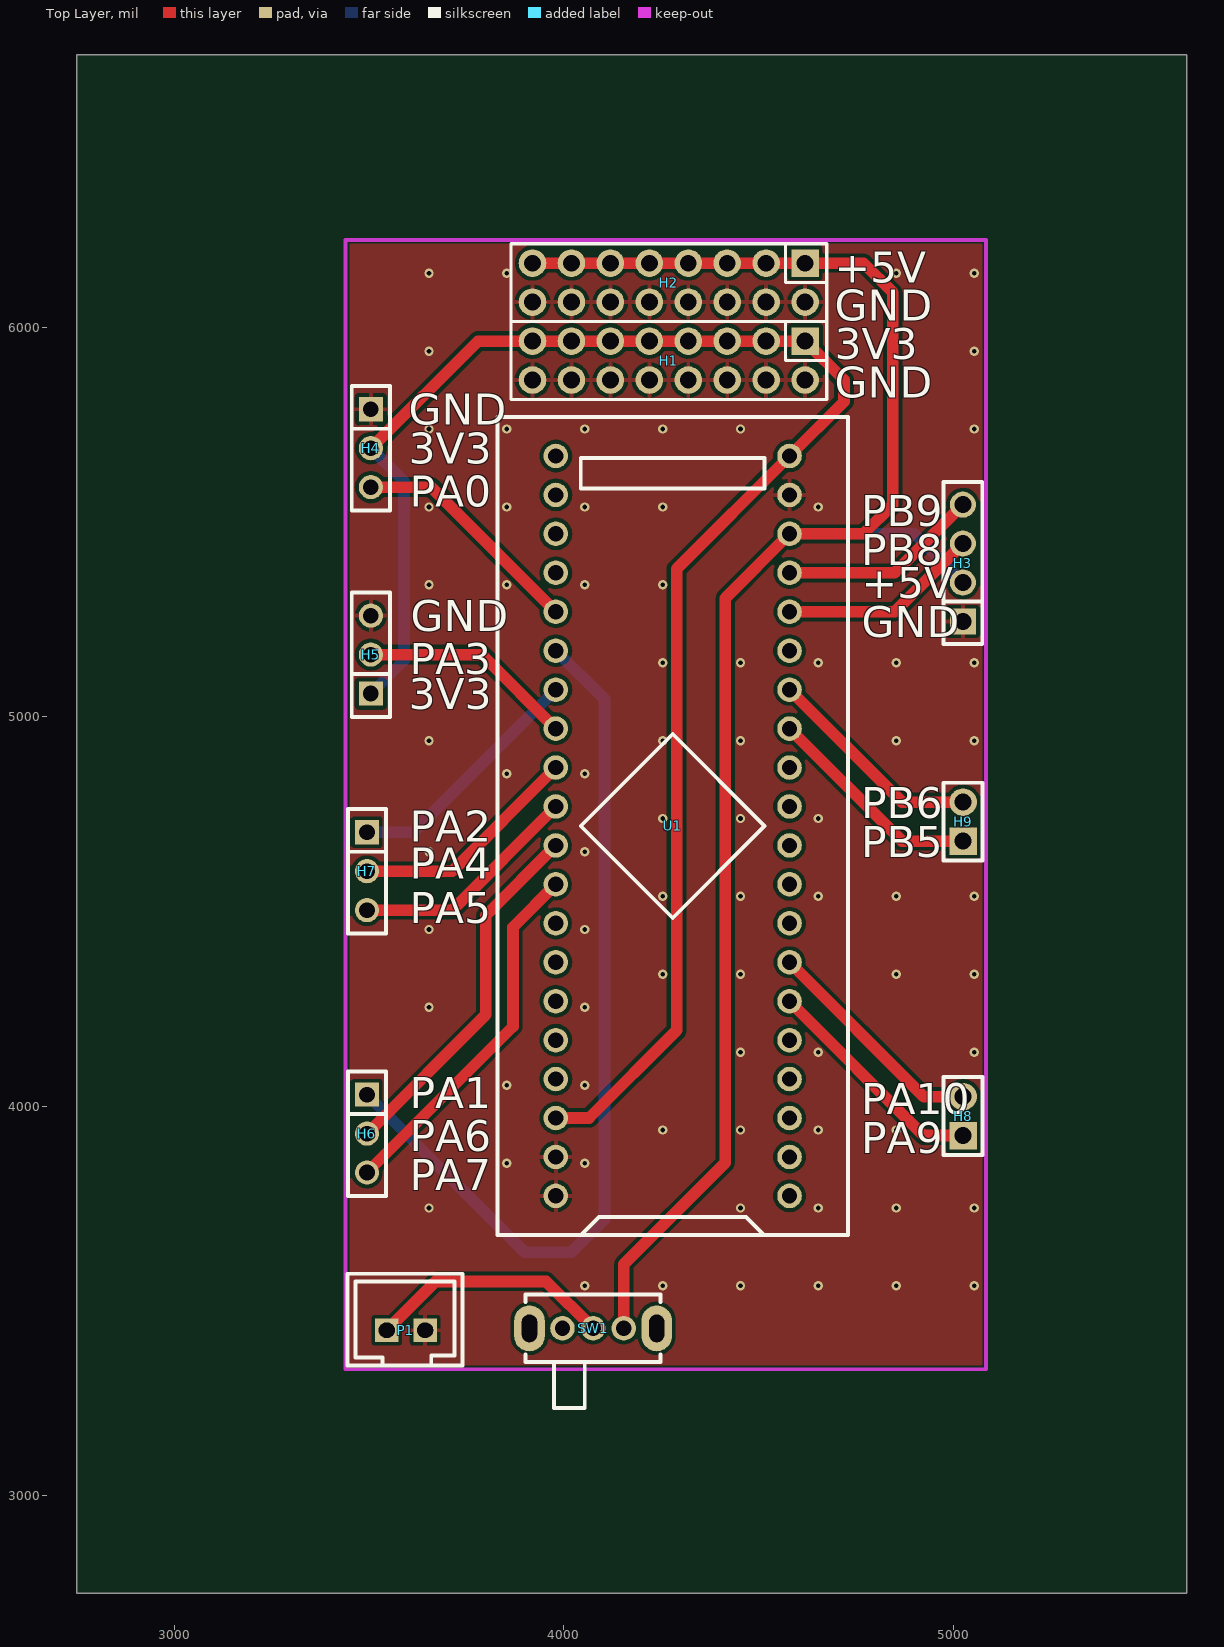
[diagram p0: Top Layer view]
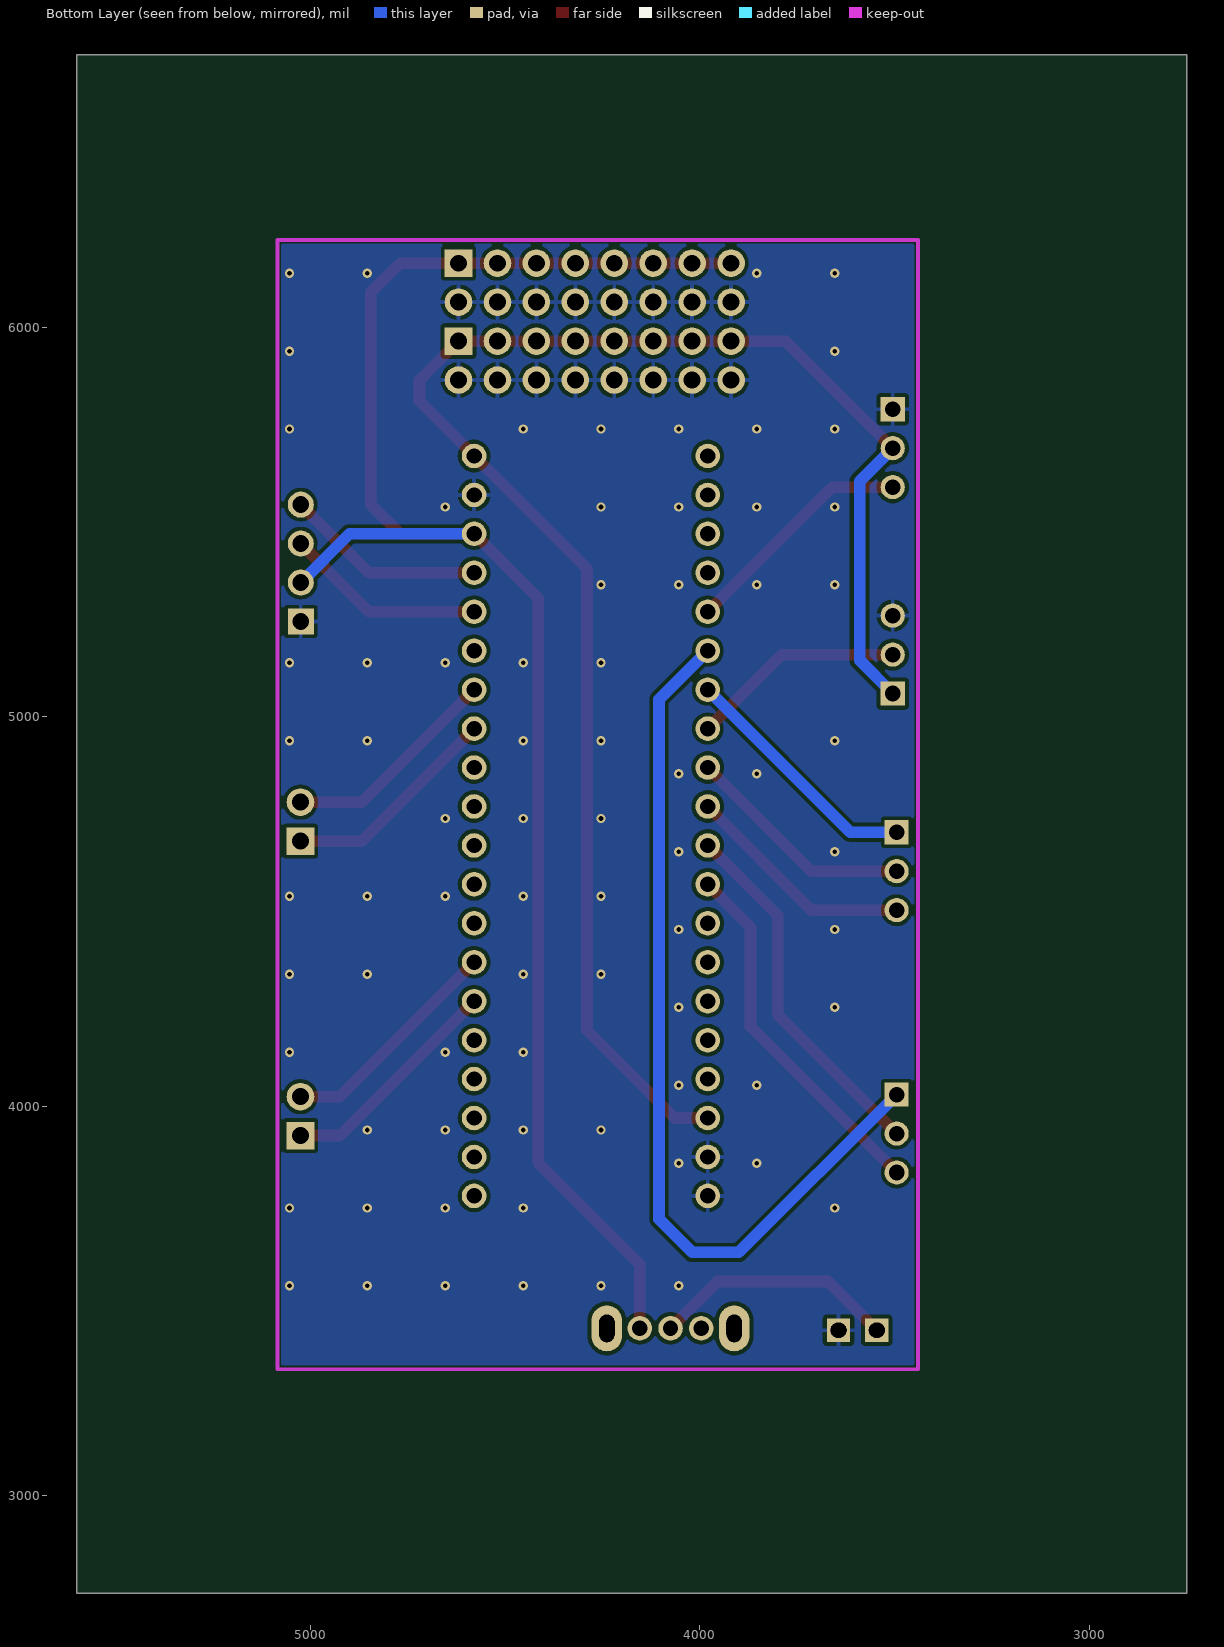
[diagram p1: Bottom Layer view, seen from below]
# Altium PCB MISC51854.pcbdoc
Units mil, origin at the board's own origin, x right, y up, seen from the top; angles counter-clockwise.
Board outline 2850 x 3950 mil, 2 copper layers (Top Layer, Bottom Layer), stack 62.206 mil thick; 12 components, 38 nets, 99 pads, 73 vias.

## Layer stack, top to bottom
Top Solder Mask Layer: solder mask 0.394, Dk 3.3
Top Layer: signal copper 1.379
Dielectric1: surface 59.449, FR4, Dk 4.5
Bottom Layer: signal copper 1.378
Bottom Solder Mask Layer: solder mask 0.394, Dk 3.3

## Board outline
5600,2750 2750,2750 2750,6700 5600,6700

## Design rules (kind name [scope] priority, off if disabled: settings)
BoardOutlineClearance copperThickness2oz_1 [All] p2 off: genericclearance=7.99 ignorepadtopadclearanceinfootprint=FALSE except(0: Arc-SplitContinuation Track-SplitContinuation SMDPad-SplitContinuation THPad-SplitContinuation Via-SplitContinuation Fill-SplitContinuation Region-SplitContinuation Poly-SplitContinuation Text-SplitContinuation Hole-SplitContinuation; 5.98: Arc-CutoutEdge Track-CutoutEdge SMDPad-CutoutEdge THPad-CutoutEdge Via-CutoutEdge Text-CutoutEdge; 6.9: Hole-OutlineEdge Hole-CutoutEdge; 10: Poly-OutlineEdge Poly-CutoutEdge; 11.81: Arc-OutlineEdge Track-OutlineEdge SMDPad-OutlineEdge THPad-OutlineEdge Via-OutlineEdge Fill-OutlineEdge Region-OutlineEdge Text-OutlineEdge Fill-CutoutEdge Region-CutoutEdge)
BoardOutlineClearance Plane_innerPlane_1 [All] p4 off: genericclearance=4.02 ignorepadtopadclearanceinfootprint=FALSE except(0: Arc-SplitContinuation Track-SplitContinuation SMDPad-SplitContinuation THPad-SplitContinuation Via-SplitContinuation Fill-SplitContinuation Region-SplitContinuation Poly-SplitContinuation Text-SplitContinuation Hole-SplitContinuation; 5.98: Arc-CutoutEdge Track-CutoutEdge SMDPad-CutoutEdge THPad-CutoutEdge Via-CutoutEdge Text-CutoutEdge; 6.9: Hole-OutlineEdge Hole-CutoutEdge; 10: Poly-OutlineEdge Poly-CutoutEdge; 11.81: Arc-OutlineEdge Track-OutlineEdge SMDPad-OutlineEdge THPad-OutlineEdge Via-OutlineEdge Fill-OutlineEdge Region-OutlineEdge Text-OutlineEdge Fill-CutoutEdge Region-CutoutEdge)
BoardOutlineClearance Copper_copperRegion_1 [All] p6 off: genericclearance=4.02 ignorepadtopadclearanceinfootprint=FALSE except(0: Arc-SplitContinuation Track-SplitContinuation SMDPad-SplitContinuation THPad-SplitContinuation Via-SplitContinuation Fill-SplitContinuation Region-SplitContinuation Poly-SplitContinuation Text-SplitContinuation Hole-SplitContinuation; 5.98: Arc-CutoutEdge Track-CutoutEdge SMDPad-CutoutEdge THPad-CutoutEdge Via-CutoutEdge Text-CutoutEdge; 6.9: Hole-OutlineEdge Hole-CutoutEdge; 10: Poly-OutlineEdge Poly-CutoutEdge; 11.81: Arc-OutlineEdge Track-OutlineEdge SMDPad-OutlineEdge THPad-OutlineEdge Via-OutlineEdge Fill-OutlineEdge Region-OutlineEdge Text-OutlineEdge Fill-CutoutEdge Region-CutoutEdge)
BoardOutlineClearance copperThickness1oz_1 [All] p8: genericclearance=4.02 ignorepadtopadclearanceinfootprint=FALSE except(0: Arc-SplitContinuation Track-SplitContinuation SMDPad-SplitContinuation THPad-SplitContinuation Via-SplitContinuation Fill-SplitContinuation Region-SplitContinuation Poly-SplitContinuation Text-SplitContinuation Hole-SplitContinuation; 5.98: Arc-CutoutEdge Track-CutoutEdge SMDPad-CutoutEdge THPad-CutoutEdge Via-CutoutEdge Text-CutoutEdge; 6.9: Hole-OutlineEdge Hole-CutoutEdge; 10: Poly-OutlineEdge Poly-CutoutEdge; 11.81: Arc-OutlineEdge Track-OutlineEdge SMDPad-OutlineEdge THPad-OutlineEdge Via-OutlineEdge Fill-OutlineEdge Region-OutlineEdge Text-OutlineEdge Fill-CutoutEdge Region-CutoutEdge)
Clearance copperThickness2oz [All] p1 off: gap=7.99 ignorepadtopadclearanceinfootprint=FALSE except(5.98: SMDPad-Track SMDPad-SMDPad THPad-Track SMDPad-THPad THPad-THPad Track-Via SMDPad-Via THPad-Via Via-Via Fill-SMDPad Region-SMDPad Fill-THPad Region-THPad Fill-Via Region-Via Fill-Fill Fill-Region Region-Region Arc-Track Arc-SMDPad Arc-THPad Arc-Via Fill-Arc Region-Arc Arc-Arc Text-Track SMDPad-Text Text-THPad Text-Via Fill-Text Region-Text Arc-Text Text-Text; 6.9: Hole-Track Hole-SMDPad Hole-THPad Hole-Via Fill-Hole Region-Hole Hole-Arc Hole-Text; 10: Poly-Track Poly-SMDPad Poly-THPad Poly-Via Poly-Fill Poly-Region Poly-Poly Poly-Arc Poly-Text Poly-Hole; 11.81: Fill-Track Region-Track)
Clearance Plane_innerPlane [All] p3 off: gap=4.02 ignorepadtopadclearanceinfootprint=FALSE except(5.98: SMDPad-Track SMDPad-SMDPad THPad-Track SMDPad-THPad THPad-THPad Track-Via SMDPad-Via THPad-Via Via-Via Fill-SMDPad Region-SMDPad Fill-THPad Region-THPad Fill-Via Region-Via Fill-Fill Fill-Region Region-Region Arc-Track Arc-SMDPad Arc-THPad Arc-Via Fill-Arc Region-Arc Arc-Arc Text-Track SMDPad-Text Text-THPad Text-Via Fill-Text Region-Text Arc-Text Text-Text; 6.9: Hole-Track Hole-SMDPad Hole-THPad Hole-Via Fill-Hole Region-Hole Hole-Arc Hole-Text; 10: Poly-Track Poly-SMDPad Poly-THPad Poly-Via Poly-Fill Poly-Region Poly-Poly Poly-Arc Poly-Text Poly-Hole; 11.81: Fill-Track Region-Track)
Clearance Copper_copperRegion [All] p5 off: gap=4.02 ignorepadtopadclearanceinfootprint=FALSE except(5.98: SMDPad-Track SMDPad-SMDPad THPad-Track SMDPad-THPad THPad-THPad Track-Via SMDPad-Via THPad-Via Via-Via Fill-SMDPad Region-SMDPad Fill-THPad Region-THPad Fill-Via Region-Via Fill-Fill Fill-Region Region-Region Arc-Track Arc-SMDPad Arc-THPad Arc-Via Fill-Arc Region-Arc Arc-Arc Text-Track SMDPad-Text Text-THPad Text-Via Fill-Text Region-Text Arc-Text Text-Text; 6.9: Hole-Track Hole-SMDPad Hole-THPad Hole-Via Fill-Hole Region-Hole Hole-Arc Hole-Text; 10: Poly-Track Poly-SMDPad Poly-THPad Poly-Via Poly-Fill Poly-Region Poly-Poly Poly-Arc Poly-Text Poly-Hole; 11.81: Fill-Track Region-Track)
Clearance copperThickness1oz [All] p7: gap=4.02 ignorepadtopadclearanceinfootprint=FALSE except(5.98: SMDPad-Track SMDPad-SMDPad THPad-Track SMDPad-THPad THPad-THPad Track-Via SMDPad-Via THPad-Via Via-Via Fill-SMDPad Region-SMDPad Fill-THPad Region-THPad Fill-Via Region-Via Fill-Fill Fill-Region Region-Region Arc-Track Arc-SMDPad Arc-THPad Arc-Via Fill-Arc Region-Arc Arc-Arc Text-Track SMDPad-Text Text-THPad Text-Via Fill-Text Region-Text Arc-Text Text-Text; 6.9: Hole-Track Hole-SMDPad Hole-THPad Hole-Via Fill-Hole Region-Hole Hole-Arc Hole-Text; 10: Poly-Track Poly-SMDPad Poly-THPad Poly-Via Poly-Fill Poly-Region Poly-Poly Poly-Arc Poly-Text Poly-Hole; 11.81: Fill-Track Region-Track)
DiffPairsRouting differentialPair [All] p1: maxlimit=6 minlimit=6 mostfreqgap=6 toplayer_minwidth=5 toplayer_prefwidth=10 toplayer_maxwidth=100 toplayer_mingap=6 toplayer_prefgap=6 toplayer_maxgap=6 bottomlayer_minwidth=5 bottomlayer_prefwidth=10 bottomlayer_maxwidth=100 bottomlayer_mingap=6 bottomlayer_prefgap=6 bottomlayer_maxgap=6 maxuncoupledlength=10
HoleToHoleClearance otherClearance [All] p1: gap=11.81 allowstackedmicrovias=TRUE
Length netLength [All] p1: minlimit=0 maxlimit=0
PasteMaskExpansion pasteMaskExpansion [All] p1: expansion=0
PlaneConnect innerPlane [All] p1: planeconnectstyle=Relief reliefexpansion=20 reliefentries=4 reliefconductorwidth=10 reliefairgap=10
PolygonConnect copperRegion [All] p1: connectstyle=Relief reliefconductorwidth=10 reliefentries=4 polygonreliefangle="90 Angle" airgapwidth=10 via.connectstyle=Relief via.reliefconductorwidth=10 via.reliefentries=4 via.polygonreliefangle="90 Angle" via.airgapwidth=10
RoutingVias viaSize [All] p1: holewidth=12.01 width=24.02 viastyle="Through Hole" minholewidth=11.81 minwidth=19.68 maxholewidth=248.03 maxwidth=393.7
SolderMaskExpansion solderMaskExpansion [IsVia] p1: expansion=-1000 istentingtop=TRUE
SolderMaskExpansion solderMaskExpansion [All] p2: expansion=2 istentingtop=FALSE
Width copperThickness2oz_2 [All] p1 off: maxlimit=100 minlimit=8 preferedwidth=10
Width copperThickness1oz_2 [All] p2: maxlimit=100 minlimit=5 preferedwidth=10

## Components (designator, comment, footprint, x,y, rotation, side; value= is the part's Value field where it differs from the comment)
H1 "" HDR-TH_16P-P2.54-V-F-R2-C8-S2.54-1 4270,5915 r180 top
H2 "" HDR-TH_16P-P2.54-V-F-R2-C8-S2.54-1 4270,6115 r180 top
H3 "" HDR-TH_4P-P2.54-V-F 5025,5395 r90 top
H4 "" HDR-TH_3P-P2.54-V-F 3505,5690 r270 top
H5 "" HDR-TH_3P-P2.54-V-F 3505,5160 r90 top
H6 "" HDR-TH_3P-P2.54-V-F 3495,3930 r270 top
H7 "" HDR-TH_3P-P2.54-V-F 3495,4603.81 r270 top
H8 "" HDR-TH_2P-P2.54-V-M-1 5025.79,3974.94 r90 top
H9 "" HDR-TH_2P-P2.54-V-M-1 5025.79,4731.03 r90 top
P1 "XH2.54直插座-2P" CONN-TH_XH2.54-2P 3595,3425 r0 top
SW1 "" 拨动开关_侧 4075.57,3429.94 r0 top
U1 "STM32F103C8T6-Card" CONN-TH_L53.3-W22.9_STM32F103C8T6-CARD 4280,4720 r90 top

## Footprints (in the part's own frame and the unit in brackets; to place one, negate y for a bottom-side part, rotate by r counter-clockwise, add the part's x,y. Pads: shape width x height; smd on the part's side, far side on the other; paste and mask are expansions set on the pad)
CONN-TH_L53.3-W22.9_STM32F103C8T6-CARD [mm]
  round 1.6 hole 1: 1(-24.13,-7.62) 2(-21.59,-7.62) 3(-19.05,-7.62) 4(-16.51,-7.62) 5(-13.97,-7.62) 6(-11.43,-7.62) 7(-8.89,-7.62) 8(-6.35,-7.62) 9(-3.81,-7.62) 10(-1.27,-7.62) 11(1.27,-7.62) 12(3.81,-7.62) 13(6.35,-7.62) 14(8.89,-7.62) 15(11.43,-7.62) 16(13.97,-7.62) 17(16.51,-7.62) 18(19.05,-7.62) 19(21.59,-7.62) 20(24.13,-7.62) 21(24.13,7.62) 22(21.59,7.62) 23(19.05,7.62) 24(16.51,7.62) 25(13.97,7.62) 26(11.43,7.62) 27(8.89,7.62) 28(6.35,7.62) 29(3.81,7.62) 30(1.27,7.62) 31(-1.27,7.62) 32(-3.81,7.62) 33(-6.35,7.62) 34(-8.89,7.62) 35(-11.43,7.62) 36(-13.97,7.62) 37(-16.51,7.62) 38(-19.05,7.62) 39(-21.59,7.62) 40(-24.13,7.62)
  silkscreen extent -26.67,-11.43 26.67,11.43
CONN-TH_XH2.54-2P [mil]
  rect 60x60 hole 39.37 slot 41.34 at 0 deg paste+0 mask+1.97: 1(-49.22,0) 2(49.21,0)
  silkscreen extent -150,-90 145,145
HDR-TH_2P-P2.54-V-M-1 [mm]
  rect 1.8x1.8 hole 1.1: 1(-1.27,0)
  round 1.8 hole 1.1: 2(1.27,0)
  silkscreen extent -2.54,-1.27 2.54,1.27
HDR-TH_3P-P2.54-V-F [mil]
  rect 62x62 hole 40.16: 1(-100,0)
  round 62 hole 40.16: 2(0,0) 3(100,0)
  silkscreen extent -160,-49 160,49
HDR-TH_4P-P2.54-V-F [mm]
  rect 1.7x1.7 hole 1.1: 1(-3.81,0)
  round 1.7 hole 1.1: 2(-1.27,0) 3(1.27,0) 4(3.81,0)
  silkscreen extent -5.29,-1.27 5.29,1.27
HDR-TH_16P-P2.54-V-F-R2-C8-S2.54-1 [mm]
  rect 1.8x1.8 hole 1.1: 1(-8.89,-1.27)
  round 1.8 hole 1.1: 2(-8.89,1.27) 3(-6.35,-1.27) 4(-6.35,1.27) 5(-3.81,-1.27) 6(-3.81,1.27) 7(-1.27,-1.27) 8(-1.27,1.27) 9(1.27,-1.27) 10(1.27,1.27) 11(3.81,-1.27) 12(3.81,1.27) 13(6.35,-1.27) 14(6.35,1.27) 15(8.89,-1.27) 16(8.89,1.27)
  silkscreen extent -10.3,-2.54 10.3,2.54
拨动开关_侧 [mil]
  round 63 hole 39.4 paste+0 mask+2: 1(-78.7,0) 2(0,0) 3(78.7,0)
  oval 78.7x118.1 hole 39.4 slot 70.9 at 90 deg paste+0 mask+2: 4(163.4,0) 5(-163.4,0)
  silkscreen extent -173,-205 173,87

## Via types
v1: diameter 24.02, hole 12, Top Layer to Bottom Layer, 73 vias

## Nets (pads, with @x,y where several pads share a name; then routed paths per layer and width w, separated by ;. In a path a pad name is that pad's centre, name@x,y a point inside that pad or via, vN(x,y) a via of type N, cw(c..) or ccw(c..) an arc to the next point about the centre after c; other vN are vias at no path point)
$1N17077: P1.1 SW1.2 | length 631.3
  Top Layer w30: P1.1 3670.78,3550 3955.51,3550 SW1.2
+5V: H2.1 H2.3 H2.5 H2.7 H2.9 H2.11 H2.13 H2.15 H3.2 SW1.3 U1.18 | length 4510.3
  Top Layer w30: H2.15 H2.13 H2.11 H2.9 H2.7 H2.5 H2.3 H2.1 4770,6165 4845,6090 4845,5545 4770,5470 U1.18 4415,5305 4415,3855 4154.27,3594.27 SW1.3
  Bottom Layer w30: U1.18 4900,5470 H3.2
GND: H1.2 H1.4 H1.6 H1.8 H1.10 H1.12 H1.14 H1.16 H2.2 H2.4 H2.6 H2.8 H2.10 H2.12 H2.14 H2.16 H3.1 H4.1 H5.3 P1.2 U1.19 U1.39 U1.40
  other v1: 4054.1,3539.1 4254.1,3539.1 4454.1,3539.1 4654.1,3539.1 4854.1,3539.1 5054.1,3539.1 3654.1,3739.1 4454.1,3739.1 4654.1,3739.1 4854.1,3739.1 5054.1,3739.1 3854.1,3854.1 4054.1,3854.1 4254.1,3939.1 4454.1,3939.1 4654.1,3939.1 4854.1,3939.1 3854.1,4054.1 4054.1,4054.1 4454.1,4139.1 4654.1,4139.1 5054.1,4139.1 3654.1,4254.1 4054.1,4254.1 4254.1,4339.1 4454.1,4339.1 4854.1,4339.1 5054.1,4339.1 3654.1,4454.1 4054.1,4454.1 4254.1,4539.1 4454.1,4539.1 4654.1,4539.1 4854.1,4539.1 5054.1,4539.1 3654.1,4654.1 4054.1,4654.1 4254.1,4739.1 4454.1,4739.1 4654.1,4739.1 3854.1,4854.1 4054.1,4854.1 3654.1,4939.1 4254.1,4939.1 4454.1,4939.1 4854.1,4939.1 5054.1,4939.1 4254.1,5139.1 4454.1,5139.1 4654.1,5139.1 4854.1,5139.1 5054.1,5139.1 3654.1,5339.1 3854.1,5339.1 4054.1,5339.1 4254.1,5339.1 3654.1,5539.1 3854.1,5539.1 4054.1,5539.1 4254.1,5539.1 4654.1,5539.1 3654.1,5739.1 3854.1,5739.1 4054.1,5739.1 4254.1,5739.1 4454.1,5739.1 5054.1,5739.1 3654.1,5939.1 5054.1,5939.1 3654.1,6139.1 3854.1,6139.1 4854.1,6139.1 5054.1,6139.1
NRST: U1.37
PA0: H4.3 U1.25 | length 607.7
  Top Layer w30: H4.3@3504.84,5590 3660,5590 U1.25
PA1: H6.1 U1.26 | length 2324.7
  Bottom Layer w30: H6.1 3900,3625 4020,3625 4105,3710 4105,5045 U1.26
PA2: H7.1 U1.27 | length 636.7
  Bottom Layer w30: H7.1 3613.8,4703.81 U1.27
PA3: H5.2 U1.28 | length 549.7
  Top Layer w30: H5.2 3790,5160 ; 3792.86,5157.14 U1.28
PA4: H7.2 U1.29 | length 595.3
  Top Layer w30: H7.2 3713.8,4603.81 U1.29
PA5: H7.3 U1.30 | length 595.3
  Top Layer w30: H7.3 3713.8,4503.81 U1.30
PA6: H6.2 U1.31 | length 940.9
  Top Layer w30: H6.2 3800,4235 3800,4490 U1.31
PA7: H6.3 U1.32 | length 940.9
  Top Layer w30: H6.3 3870,4205 3870,4460 U1.32
PA8: U1.5
PA9: H8.1 U1.6 | length 588.7
  Top Layer w30: U1.6 4925.06,3924.94 H8.1
PA10: H8.2 U1.7 | length 588.7
  Top Layer w30: U1.7 4925.06,4024.94 H8.2
PA11: U1.8
PA12: U1.9
PA15: U1.10
PB0: U1.33
PB1: U1.34
PB3: U1.11
PB4: U1.12
PB5: H9.1 U1.13 | length 565.5
  Top Layer w30: U1.13 4868.97,4681.03 H9.1
PB6: H9.2 U1.14 | length 565.5
  Top Layer w30: U1.14 4868.97,4781.03 H9.2
PB7: U1.15
PB8: H3.3 U1.16 | length 517.5
  Top Layer w30: U1.16 4850,5270 H3.3
PB9: H3.4 U1.17 | length 517.5
  Top Layer w30: U1.17 4850,5370 H3.4
PB10: U1.35
PB11: U1.36
PB12: U1.1
PB13: U1.2
PB14: U1.3
PB15: U1.4
PC13: U1.22
PC14: U1.23
PC15: U1.24
VBAT: U1.21
VCC: H1.1 H1.3 H1.5 H1.7 H1.9 H1.11 H1.13 H1.15 H4.2 H5.1 U1.20 U1.38 | length 4322.1
  Top Layer w30: H4.2 3780,5965 H1.15 H1.13 H1.11 H1.9 H1.7 H1.5 H1.3 H1.1 4720,5865 4720,5810 U1.20 4290,5380 4290,4195 4065,3970 U1.38
  Bottom Layer w30: H5.1 3590,5145 3590,5605 H4.2
pads on no net: SW1.1 SW1.4 SW1.5

## Polygon pours and split planes (outlines as drawn)
GND on Top Layer (solid, remove dead copper, pour order 0): 3000,6450 3000,3000 5350,3000 5350,6450
GND on Bottom Layer (solid, remove dead copper, pour order 2): 3135,6315 3135,3130 5260,3130 5260,6315

## Keep-outs
Board Outline Layer:
  lines w10: 3440,3325 3440,6225 5085,6225 5085,3325 3440,3325

## Silkscreen, mask and mechanical layers (free items; w line width, h text height)
Top Silkscreen Layer:
  text "+5V" at 4695.95,6115 h80
  text "GND" at 4695.95,6016.67 h80
  text "3V3" at 4695.95,5918.33 h80
  text "GND" at 4695.95,5820 h80
  text "GND" at 3602.7,5750 h80
  text "3V3" at 3602.7,5650 h80
  text "PA0" at 3605,5540 h80
  text "PB9" at 4764.16,5490 h80
  text "PB8" at 4764.16,5390 h80
  text "+5V" at 4765,5305 h80
  text "GND" at 3607.7,5220 h80
  text "GND" at 4764.95,5205 h80
  text "PA3" at 3605,5110 h80
  text "3V3" at 3602.7,5020 h80
  text "PB6" at 4764.16,4740 h80
  text "PA2" at 3605,4680 h80
  text "PB5" at 4764.16,4640 h80
  text "PA4" at 3605,4585 h80
  text "PA5" at 3605,4470 h80
  text "PA1" at 3605,3995 h80
  text "PA10" at 4764.16,3980 h80
  text "PA6" at 3605,3885 h80
  text "PA9" at 4764.16,3880 h80
  text "PA7" at 3605,3785 h80